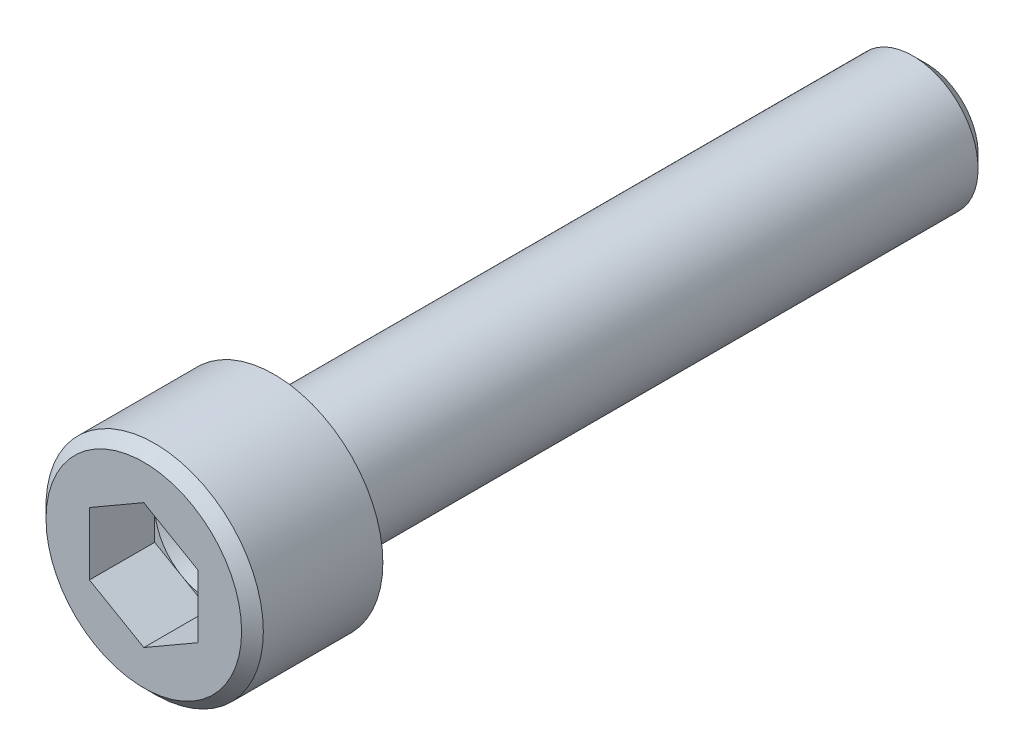
SolidWorks part; units mm, degrees
material "SUS304/0Cr18Ni9"
ref_plane "前视基准面" through (0, 0, 0) normal (0, 0, 1) x (1, 0, 0)
ref_plane "上视基准面" through (0, 0, 0) normal (0, 1, 0) x (1, 0, 0)
ref_plane "右视基准面" through (0, 0, 0) normal (1, 0, 0) x (0, 0, -1)
sketch "草图1" plane through (0, 0, 0) normal (0, 1, 0) x (1, 0, 0)
  line L0 (5, 0) -> (0, 0)
  line L1 (0, 0) -> (0, -6)
  line L2 (0, -6) -> (5, -6)
  line L3 (5, -6) -> (5, 0)
  line L4 (0, 0) -> (0, -6) construction
revolve "旋转1" add sketch "草图1" angle 360 about L4
sketch "草图2" plane through (0, 0, 0) normal (0, 0, -1) x (-1, 0, 0)
  circle A0 centre (0, 0) radius 3
extrude "凸台-拉伸1" add sketch "草图2" along normal blind 30
sketch "草图3" plane through (0, 0, 6) normal (0, 0, 1) x (1, 0, 0)
  line L0 (2.5, 1.4434) -> (0, 2.8868)
  line L1 (0, 2.8868) -> (-2.5, 1.4434)
  line L2 (-2.5, 1.4434) -> (-2.5, -1.4434)
  line L3 (-2.5, -1.4434) -> (0, -2.8868)
  line L4 (0, -2.8868) -> (2.5, -1.4434)
  line L5 (2.5, -1.4434) -> (2.5, 1.4434)
extrude "切除-拉伸1" cut sketch "草图3" against normal blind 3
ref_plane "基准面1" through (0, 0, 0) normal (0, -1, 0) x (1, 0, 0)
sketch "草图4" plane through (0, 0, 0) normal (0, -1, 0) x (1, 0, 0)
  line L0 (2.5, 3) -> (0, 3)
  line L1 (0, 3) -> (0, 1.5566)
  line L2 (0, 1.5566) -> (2.5, 3)
  line L3 (0, 3) -> (0, 1.5566) construction
revolve "切除-旋转1" cut sketch "草图4" angle 360 about L3
chamfer "倒角1" distance 0.5 angle 45 1 edges at (5, 0, 6)
chamfer "倒角2" distance 0.6135 angle 45 1 edges at (-3, 0, -30)
